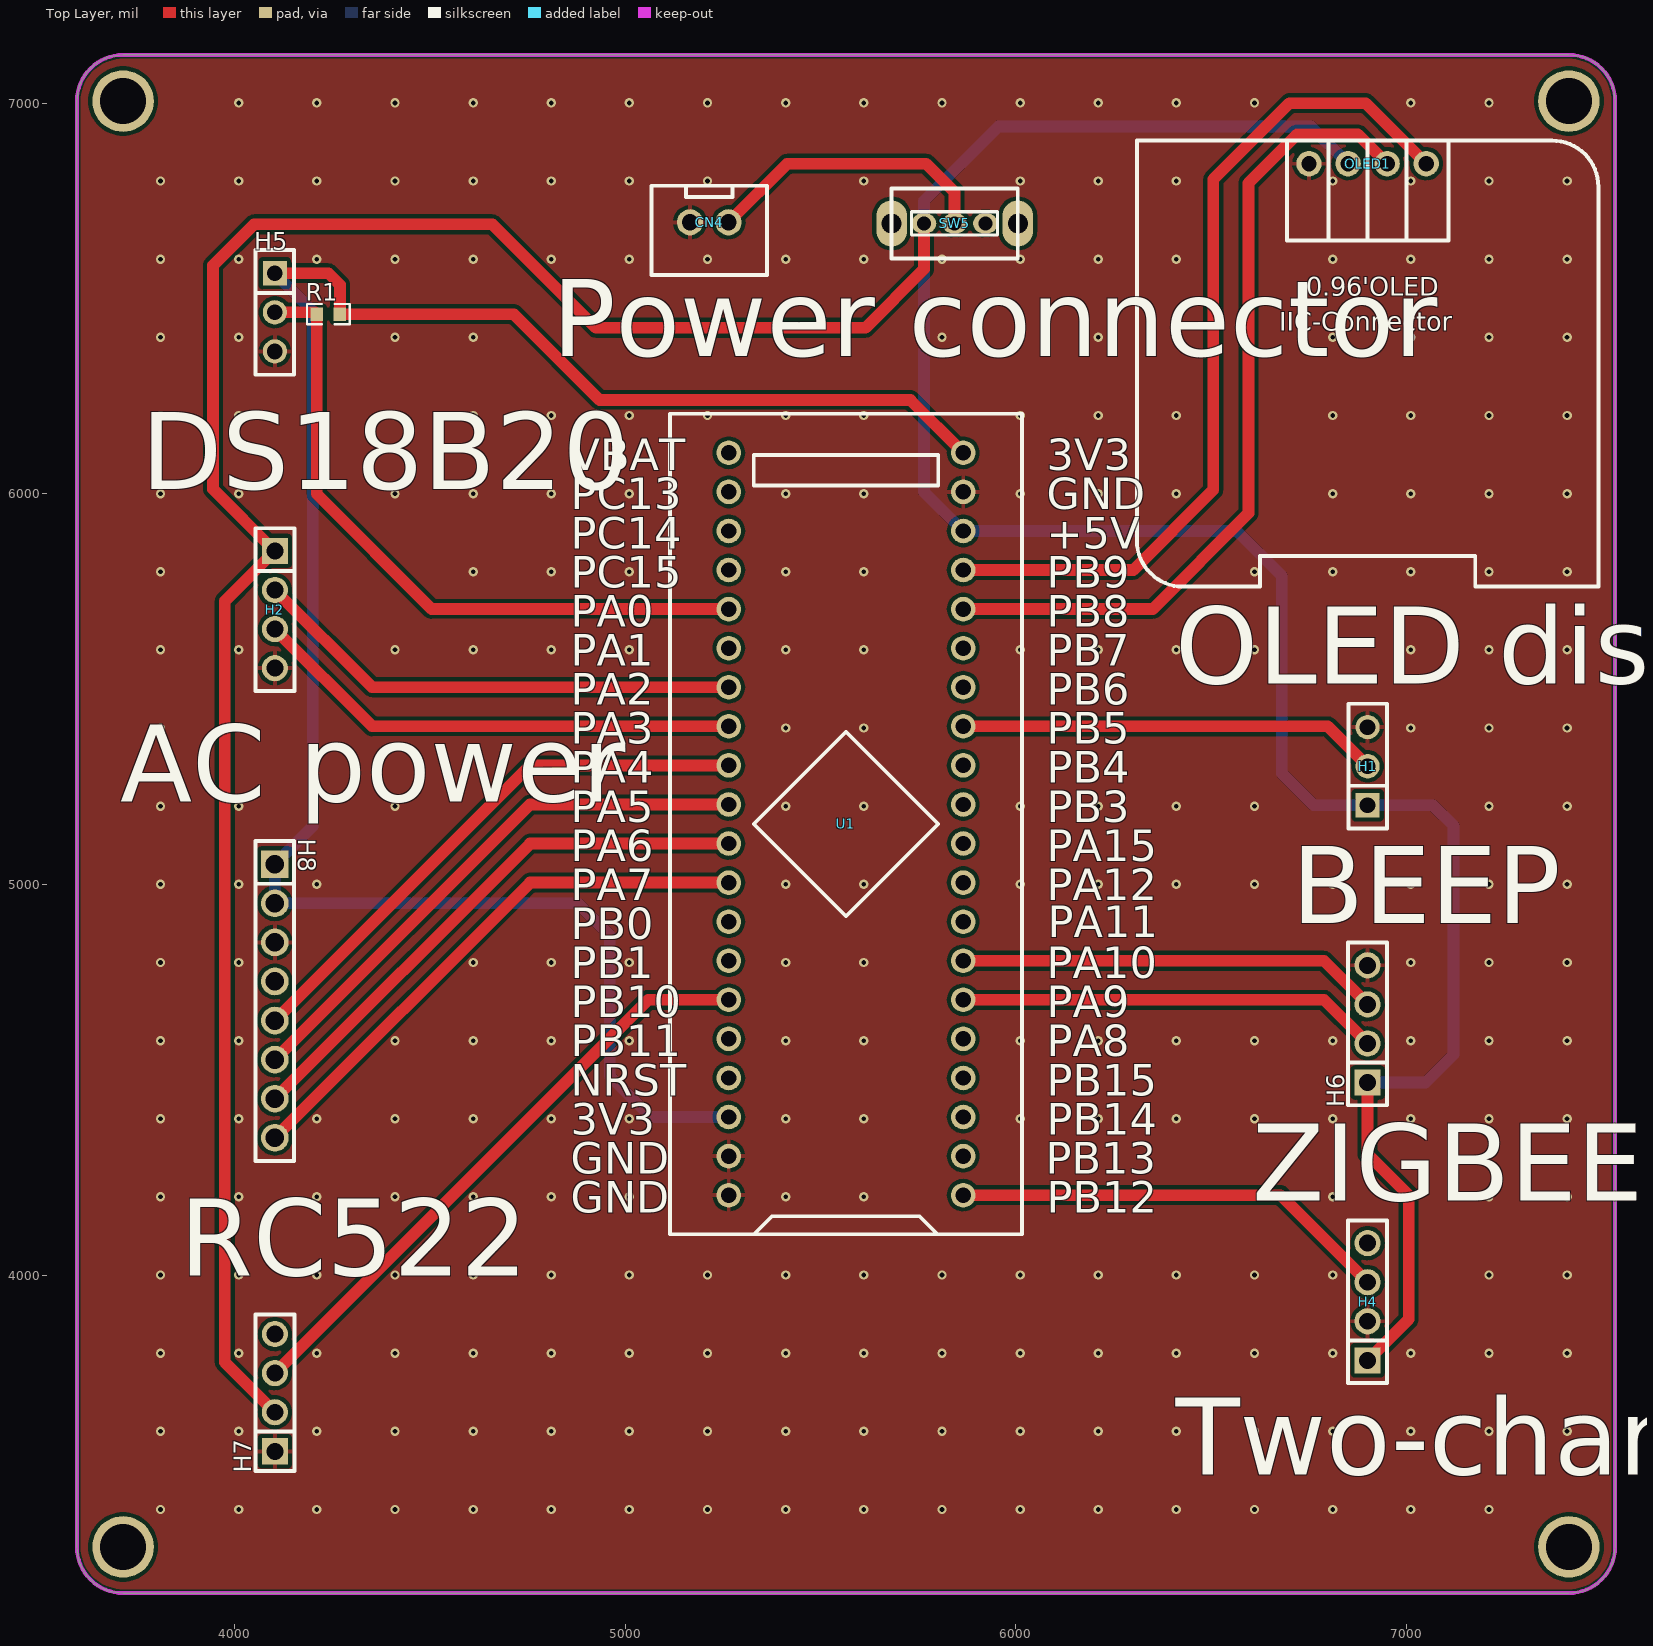
[diagram p0: Top Layer view]
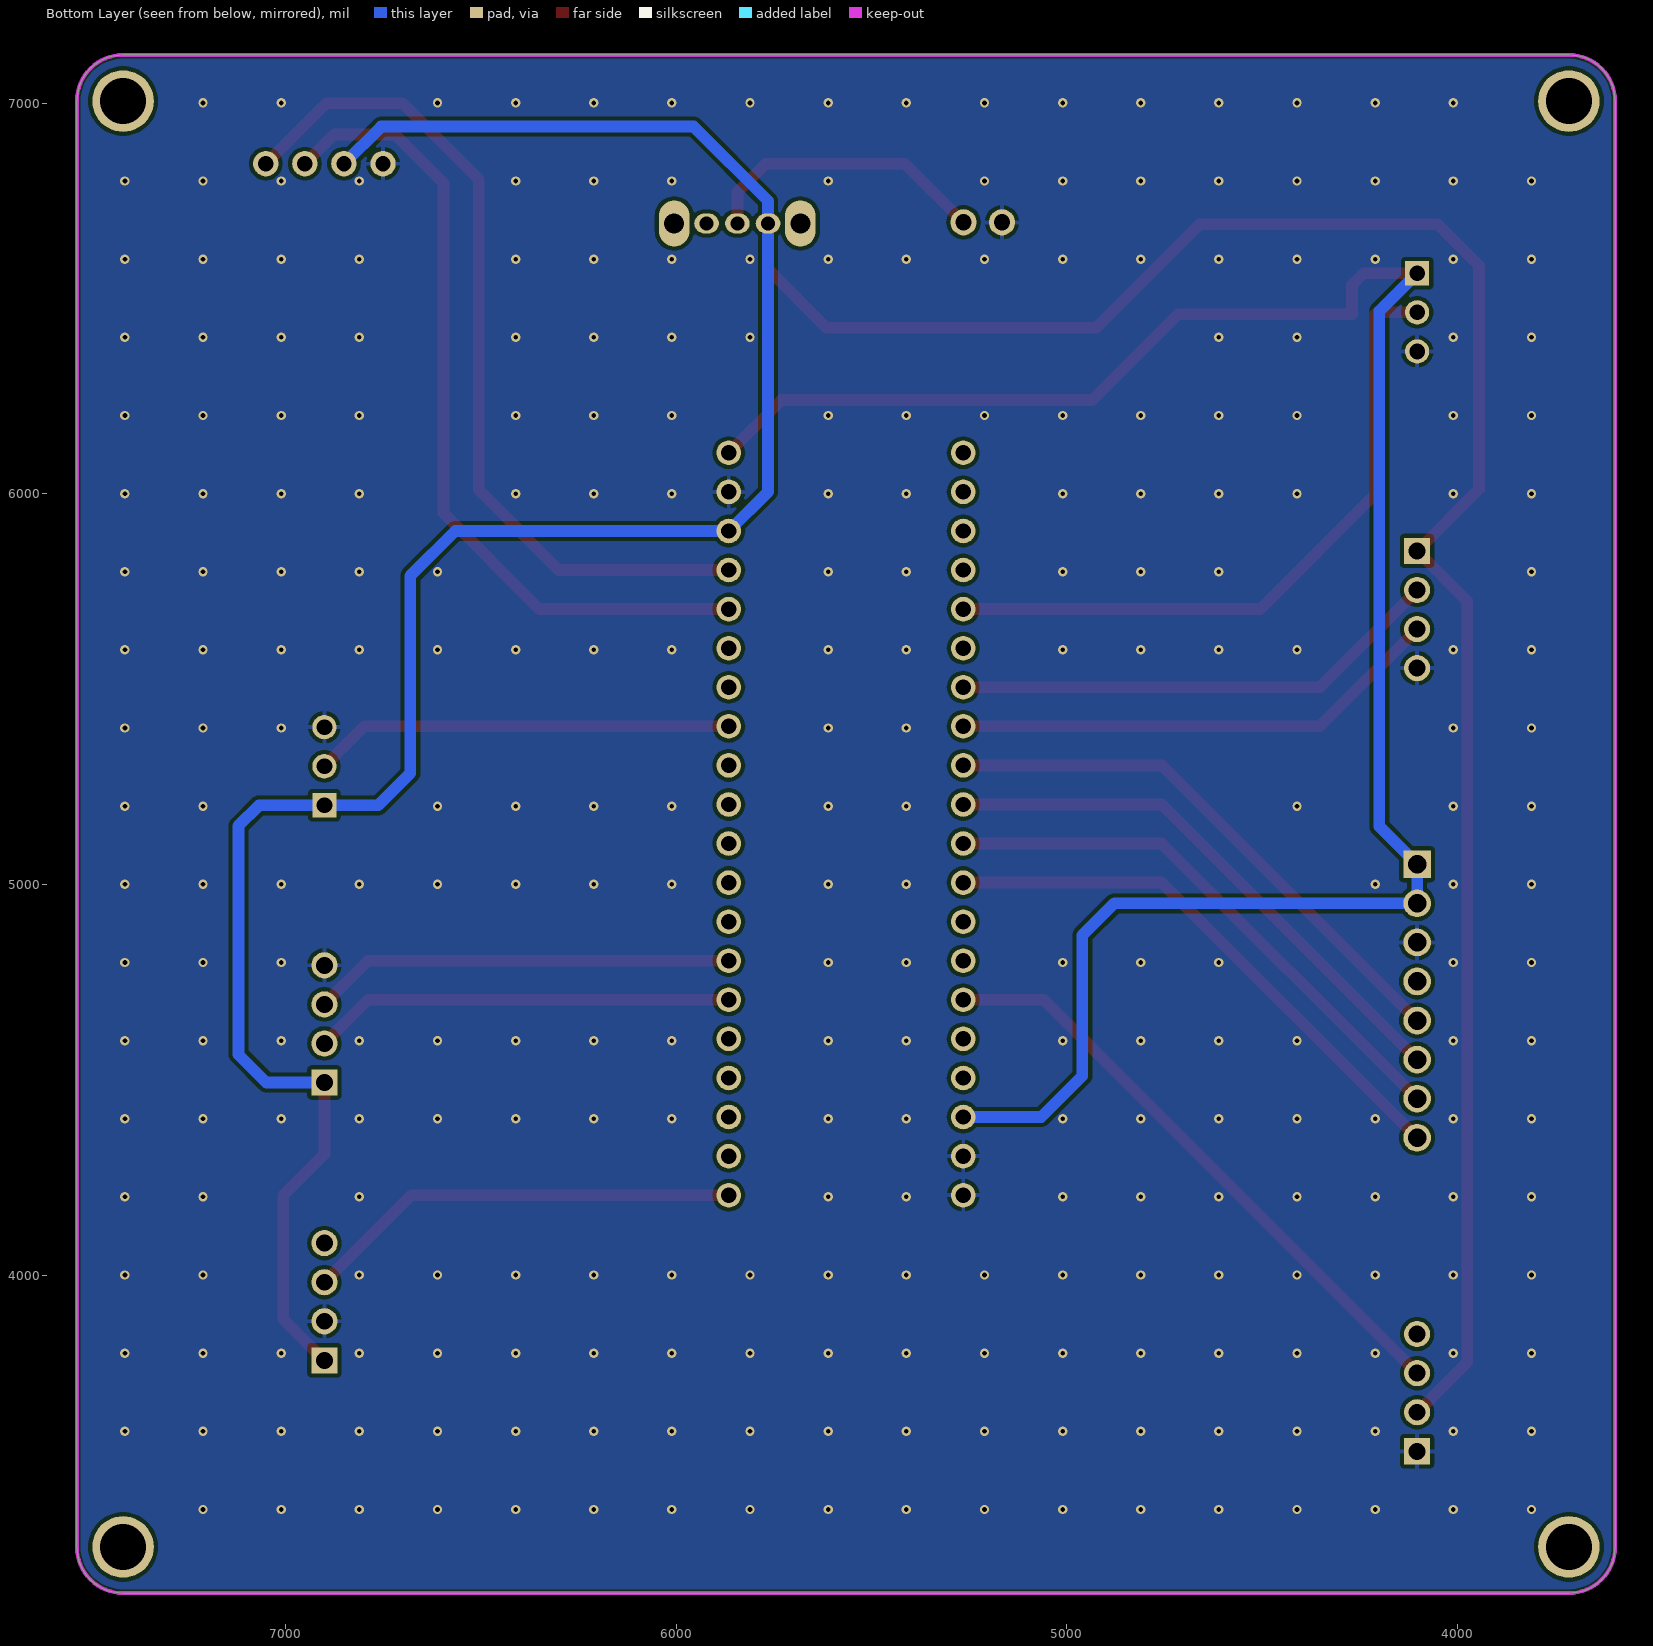
[diagram p1: Bottom Layer view, seen from below]
# Altium PCB MISC88997.pcbdoc
Units mil, origin at the board's own origin, x right, y up, seen from the top; angles counter-clockwise.
Board outline 3937.01 x 3937.01 mil, 2 copper layers (Top Layer, Bottom Layer), stack 62.206 mil thick; 12 components, 38 nets, 87 pads, 280 vias.

## Layer stack, top to bottom
Top Solder Mask Layer: solder mask 0.394, Dk 3.3
Top Layer: signal copper 1.379
Dielectric1: surface 59.449, FR4, Dk 4.5
Bottom Layer: signal copper 1.378
Bottom Solder Mask Layer: solder mask 0.394, Dk 3.3

## Board outline
3714.61,7123.5 ccw(c3714.61,7005.39) 3596.5,7005.39 3596.5,3304.61 ccw(c3714.61,3304.61) 3714.61,3186.5 7415.39,3186.5 ccw(c7415.39,3304.61) 7533.5,3304.61 7533.5,7005.39 ccw(c7415.39,7005.39) 7415.39,7123.5 3714.61,7123.5

## Design rules (kind name [scope] priority, off if disabled: settings)
BoardOutlineClearance copperThickness2oz_1 [All] p2 off: genericclearance=7.99 ignorepadtopadclearanceinfootprint=FALSE except(0: Arc-SplitContinuation Track-SplitContinuation SMDPad-SplitContinuation THPad-SplitContinuation Via-SplitContinuation Fill-SplitContinuation Region-SplitContinuation Poly-SplitContinuation Text-SplitContinuation Hole-SplitContinuation; 5.98: Arc-CutoutEdge Track-CutoutEdge SMDPad-CutoutEdge THPad-CutoutEdge Via-CutoutEdge Text-CutoutEdge; 6.9: Hole-OutlineEdge Hole-CutoutEdge; 10: Poly-OutlineEdge Poly-CutoutEdge; 11.81: Arc-OutlineEdge Track-OutlineEdge SMDPad-OutlineEdge THPad-OutlineEdge Via-OutlineEdge Fill-OutlineEdge Region-OutlineEdge Text-OutlineEdge Fill-CutoutEdge Region-CutoutEdge)
BoardOutlineClearance Plane_innerPlane_1 [All] p4 off: genericclearance=4.02 ignorepadtopadclearanceinfootprint=FALSE except(0: Arc-SplitContinuation Track-SplitContinuation SMDPad-SplitContinuation THPad-SplitContinuation Via-SplitContinuation Fill-SplitContinuation Region-SplitContinuation Poly-SplitContinuation Text-SplitContinuation Hole-SplitContinuation; 5.98: Arc-CutoutEdge Track-CutoutEdge SMDPad-CutoutEdge THPad-CutoutEdge Via-CutoutEdge Text-CutoutEdge; 6.9: Hole-OutlineEdge Hole-CutoutEdge; 10: Poly-OutlineEdge Poly-CutoutEdge; 11.81: Arc-OutlineEdge Track-OutlineEdge SMDPad-OutlineEdge THPad-OutlineEdge Via-OutlineEdge Fill-OutlineEdge Region-OutlineEdge Text-OutlineEdge Fill-CutoutEdge Region-CutoutEdge)
BoardOutlineClearance Copper_copperRegion_1 [All] p6 off: genericclearance=4.02 ignorepadtopadclearanceinfootprint=FALSE except(0: Arc-SplitContinuation Track-SplitContinuation SMDPad-SplitContinuation THPad-SplitContinuation Via-SplitContinuation Fill-SplitContinuation Region-SplitContinuation Poly-SplitContinuation Text-SplitContinuation Hole-SplitContinuation; 5.98: Arc-CutoutEdge Track-CutoutEdge SMDPad-CutoutEdge THPad-CutoutEdge Via-CutoutEdge Text-CutoutEdge; 6.9: Hole-OutlineEdge Hole-CutoutEdge; 10: Poly-OutlineEdge Poly-CutoutEdge; 11.81: Arc-OutlineEdge Track-OutlineEdge SMDPad-OutlineEdge THPad-OutlineEdge Via-OutlineEdge Fill-OutlineEdge Region-OutlineEdge Text-OutlineEdge Fill-CutoutEdge Region-CutoutEdge)
BoardOutlineClearance Copper_copperRegion_copperThickness1oz_1 [All] p8 off: genericclearance=4.02 ignorepadtopadclearanceinfootprint=FALSE except(0: Arc-SplitContinuation Track-SplitContinuation SMDPad-SplitContinuation THPad-SplitContinuation Via-SplitContinuation Fill-SplitContinuation Region-SplitContinuation Poly-SplitContinuation Text-SplitContinuation Hole-SplitContinuation; 5.98: Arc-CutoutEdge Track-CutoutEdge SMDPad-CutoutEdge THPad-CutoutEdge Via-CutoutEdge Text-CutoutEdge; 6.9: Hole-OutlineEdge Hole-CutoutEdge; 10: Poly-OutlineEdge Poly-CutoutEdge; 11.81: Arc-OutlineEdge Track-OutlineEdge SMDPad-OutlineEdge THPad-OutlineEdge Via-OutlineEdge Fill-OutlineEdge Region-OutlineEdge Text-OutlineEdge Fill-CutoutEdge Region-CutoutEdge)
BoardOutlineClearance Copper_copperRegion_Copper_copperRegion_1 [All] p10 off: genericclearance=4.02 ignorepadtopadclearanceinfootprint=FALSE except(0: Arc-SplitContinuation Track-SplitContinuation SMDPad-SplitContinuation THPad-SplitContinuation Via-SplitContinuation Fill-SplitContinuation Region-SplitContinuation Poly-SplitContinuation Text-SplitContinuation Hole-SplitContinuation; 5.98: Arc-CutoutEdge Track-CutoutEdge SMDPad-CutoutEdge THPad-CutoutEdge Via-CutoutEdge Text-CutoutEdge; 6.9: Hole-OutlineEdge Hole-CutoutEdge; 10: Poly-OutlineEdge Poly-CutoutEdge; 11.81: Arc-OutlineEdge Track-OutlineEdge SMDPad-OutlineEdge THPad-OutlineEdge Via-OutlineEdge Fill-OutlineEdge Region-OutlineEdge Text-OutlineEdge Fill-CutoutEdge Region-CutoutEdge)
BoardOutlineClearance copperThickness1oz_1 [All] p12: genericclearance=4.02 ignorepadtopadclearanceinfootprint=FALSE except(0: Arc-SplitContinuation Track-SplitContinuation SMDPad-SplitContinuation THPad-SplitContinuation Via-SplitContinuation Fill-SplitContinuation Region-SplitContinuation Poly-SplitContinuation Text-SplitContinuation Hole-SplitContinuation; 5.98: Arc-CutoutEdge Track-CutoutEdge SMDPad-CutoutEdge THPad-CutoutEdge Via-CutoutEdge Text-CutoutEdge; 6.9: Hole-OutlineEdge Hole-CutoutEdge; 10: Poly-OutlineEdge Poly-CutoutEdge; 11.81: Arc-OutlineEdge Track-OutlineEdge SMDPad-OutlineEdge THPad-OutlineEdge Via-OutlineEdge Fill-OutlineEdge Region-OutlineEdge Text-OutlineEdge Fill-CutoutEdge Region-CutoutEdge)
Clearance copperThickness2oz [All] p1 off: gap=7.99 ignorepadtopadclearanceinfootprint=FALSE except(5.98: SMDPad-Track SMDPad-SMDPad THPad-Track SMDPad-THPad THPad-THPad Track-Via SMDPad-Via THPad-Via Via-Via Fill-SMDPad Region-SMDPad Fill-THPad Region-THPad Fill-Via Region-Via Fill-Fill Fill-Region Region-Region Arc-Track Arc-SMDPad Arc-THPad Arc-Via Fill-Arc Region-Arc Arc-Arc Text-Track SMDPad-Text Text-THPad Text-Via Fill-Text Region-Text Arc-Text Text-Text; 6.9: Hole-Track Hole-SMDPad Hole-THPad Hole-Via Fill-Hole Region-Hole Hole-Arc Hole-Text; 10: Poly-Track Poly-SMDPad Poly-THPad Poly-Via Poly-Fill Poly-Region Poly-Poly Poly-Arc Poly-Text Poly-Hole; 11.81: Fill-Track Region-Track)
Clearance Plane_innerPlane [All] p3 off: gap=4.02 ignorepadtopadclearanceinfootprint=FALSE except(5.98: SMDPad-Track SMDPad-SMDPad THPad-Track SMDPad-THPad THPad-THPad Track-Via SMDPad-Via THPad-Via Via-Via Fill-SMDPad Region-SMDPad Fill-THPad Region-THPad Fill-Via Region-Via Fill-Fill Fill-Region Region-Region Arc-Track Arc-SMDPad Arc-THPad Arc-Via Fill-Arc Region-Arc Arc-Arc Text-Track SMDPad-Text Text-THPad Text-Via Fill-Text Region-Text Arc-Text Text-Text; 6.9: Hole-Track Hole-SMDPad Hole-THPad Hole-Via Fill-Hole Region-Hole Hole-Arc Hole-Text; 10: Poly-Track Poly-SMDPad Poly-THPad Poly-Via Poly-Fill Poly-Region Poly-Poly Poly-Arc Poly-Text Poly-Hole; 11.81: Fill-Track Region-Track)
Clearance Copper_copperRegion [All] p5 off: gap=4.02 ignorepadtopadclearanceinfootprint=FALSE except(5.98: SMDPad-Track SMDPad-SMDPad THPad-Track SMDPad-THPad THPad-THPad Track-Via SMDPad-Via THPad-Via Via-Via Fill-SMDPad Region-SMDPad Fill-THPad Region-THPad Fill-Via Region-Via Fill-Fill Fill-Region Region-Region Arc-Track Arc-SMDPad Arc-THPad Arc-Via Fill-Arc Region-Arc Arc-Arc Text-Track SMDPad-Text Text-THPad Text-Via Fill-Text Region-Text Arc-Text Text-Text; 6.9: Hole-Track Hole-SMDPad Hole-THPad Hole-Via Fill-Hole Region-Hole Hole-Arc Hole-Text; 10: Poly-Track Poly-SMDPad Poly-THPad Poly-Via Poly-Fill Poly-Region Poly-Poly Poly-Arc Poly-Text Poly-Hole; 11.81: Fill-Track Region-Track)
Clearance Copper_copperRegion_copperThickness1oz [All] p7 off: gap=4.02 ignorepadtopadclearanceinfootprint=FALSE except(5.98: SMDPad-Track SMDPad-SMDPad THPad-Track SMDPad-THPad THPad-THPad Track-Via SMDPad-Via THPad-Via Via-Via Fill-SMDPad Region-SMDPad Fill-THPad Region-THPad Fill-Via Region-Via Fill-Fill Fill-Region Region-Region Arc-Track Arc-SMDPad Arc-THPad Arc-Via Fill-Arc Region-Arc Arc-Arc Text-Track SMDPad-Text Text-THPad Text-Via Fill-Text Region-Text Arc-Text Text-Text; 6.9: Hole-Track Hole-SMDPad Hole-THPad Hole-Via Fill-Hole Region-Hole Hole-Arc Hole-Text; 10: Poly-Track Poly-SMDPad Poly-THPad Poly-Via Poly-Fill Poly-Region Poly-Poly Poly-Arc Poly-Text Poly-Hole; 11.81: Fill-Track Region-Track)
Clearance Copper_copperRegion_Copper_copperRegion [All] p9 off: gap=4.02 ignorepadtopadclearanceinfootprint=FALSE except(5.98: SMDPad-Track SMDPad-SMDPad THPad-Track SMDPad-THPad THPad-THPad Track-Via SMDPad-Via THPad-Via Via-Via Fill-SMDPad Region-SMDPad Fill-THPad Region-THPad Fill-Via Region-Via Fill-Fill Fill-Region Region-Region Arc-Track Arc-SMDPad Arc-THPad Arc-Via Fill-Arc Region-Arc Arc-Arc Text-Track SMDPad-Text Text-THPad Text-Via Fill-Text Region-Text Arc-Text Text-Text; 6.9: Hole-Track Hole-SMDPad Hole-THPad Hole-Via Fill-Hole Region-Hole Hole-Arc Hole-Text; 10: Poly-Track Poly-SMDPad Poly-THPad Poly-Via Poly-Fill Poly-Region Poly-Poly Poly-Arc Poly-Text Poly-Hole; 11.81: Fill-Track Region-Track)
Clearance copperThickness1oz [All] p11: gap=4.02 ignorepadtopadclearanceinfootprint=FALSE except(5.98: SMDPad-Track SMDPad-SMDPad THPad-Track SMDPad-THPad THPad-THPad Track-Via SMDPad-Via THPad-Via Via-Via Fill-SMDPad Region-SMDPad Fill-THPad Region-THPad Fill-Via Region-Via Fill-Fill Fill-Region Region-Region Arc-Track Arc-SMDPad Arc-THPad Arc-Via Fill-Arc Region-Arc Arc-Arc Text-Track SMDPad-Text Text-THPad Text-Via Fill-Text Region-Text Arc-Text Text-Text; 6.9: Hole-Track Hole-SMDPad Hole-THPad Hole-Via Fill-Hole Region-Hole Hole-Arc Hole-Text; 10: Poly-Track Poly-SMDPad Poly-THPad Poly-Via Poly-Fill Poly-Region Poly-Poly Poly-Arc Poly-Text Poly-Hole; 11.81: Fill-Track Region-Track)
DiffPairsRouting differentialPair [All] p1: maxlimit=6 minlimit=6 mostfreqgap=6 toplayer_minwidth=5 toplayer_prefwidth=10 toplayer_maxwidth=100 toplayer_mingap=6 toplayer_prefgap=6 toplayer_maxgap=6 bottomlayer_minwidth=5 bottomlayer_prefwidth=10 bottomlayer_maxwidth=100 bottomlayer_mingap=6 bottomlayer_prefgap=6 bottomlayer_maxgap=6 maxuncoupledlength=10
HoleToHoleClearance otherClearance [All] p1: gap=11.81 allowstackedmicrovias=TRUE
Length netLength [All] p1: minlimit=0 maxlimit=0
PasteMaskExpansion pasteMaskExpansion [All] p1: expansion=0
PlaneConnect innerPlane [All] p1: planeconnectstyle=Relief reliefexpansion=20 reliefentries=4 reliefconductorwidth=10 reliefairgap=10
PolygonConnect copperRegion_copperThickness1oz [All] p1 off: connectstyle=Relief reliefconductorwidth=10 reliefentries=4 polygonreliefangle="90 Angle" airgapwidth=10 via.connectstyle=Relief via.reliefconductorwidth=10 via.reliefentries=4 via.polygonreliefangle="90 Angle" via.airgapwidth=10
PolygonConnect copperRegion_Copper_copperRegion [All] p2 off: connectstyle=Relief reliefconductorwidth=10 reliefentries=4 polygonreliefangle="90 Angle" airgapwidth=10 via.connectstyle=Relief via.reliefconductorwidth=10 via.reliefentries=4 via.polygonreliefangle="90 Angle" via.airgapwidth=10
PolygonConnect copperRegion [All] p3: connectstyle=Relief reliefconductorwidth=10 reliefentries=4 polygonreliefangle="90 Angle" airgapwidth=10 via.connectstyle=Relief via.reliefconductorwidth=10 via.reliefentries=4 via.polygonreliefangle="90 Angle" via.airgapwidth=10
RoutingVias viaSize [All] p1: holewidth=12.01 width=24.02 viastyle="Through Hole" minholewidth=11.81 minwidth=19.68 maxholewidth=248.03 maxwidth=393.7
SolderMaskExpansion solderMaskExpansion [IsVia] p1: expansion=-1000 istentingtop=TRUE
SolderMaskExpansion solderMaskExpansion [All] p2: expansion=2 istentingtop=FALSE
Width copperThickness2oz_2 [All] p1 off: maxlimit=100 minlimit=8 preferedwidth=10
Width copperThickness1oz_2 [All] p2: maxlimit=100 minlimit=5 preferedwidth=10

## Components (designator, comment, footprint, x,y, rotation, side; value= is the part's Value field where it differs from the comment)
CN4 "XH2.54*2P_through-hole" CONN-TH_2P-P2.50-XH2.54-2P 5215,6695 r0 top
H1 "" HDR-TH_3P-P2.54-V-F 6900,5302.82 r90 top
H2 "" HDR-TH_4P-P2.54-V-F 4103.27,5703.79 r270 top
H4 "" HDR-TH_4P-P2.54-V-F 6900,3932.22 r90 top
H5 "" HDR-TH_3P-P2.54-V-F 4103.27,6464.57 r270 top
H6 "" HDR-TH_4P-P2.54-V-F 6900,4643.38 r90 top
H7 "" HDR-TH_4P-P2.54-V-M 4103.27,3699.44 r90 top
H8 "" HDR-TH_8P-P2.54-V-F-1 4103.27,4701.96 r270 top
OLED1 "" 0.96OLED_4P 6900,6845 r0 top
R1 "4.7K" R0603 4240,6460 r0 top
SW5 "" 拨动开关 5837.9,6692.05 r0 top
U1 "STM32F103C8T6-Card" CONN-TH_L53.3-W22.9_STM32F103C8T6-CARD 5565,5155 r90 top

## Footprints (in the part's own frame and the unit in brackets; to place one, negate y for a bottom-side part, rotate by r counter-clockwise, add the part's x,y. Pads: shape width x height; smd on the part's side, far side on the other; paste and mask are expansions set on the pad)
0.96OLED_4P [mm]
  round 1.65 hole 1 copper offset 0,0: 1(-3.81,-0.001) 2(-1.27,0.002) 3(1.27,0.002) 4(3.81,0.002)
  silkscreen extent -15,-27.5 15,1.5
CONN-TH_2P-P2.50-XH2.54-2P [mm]
  round 1.7 hole 1.05 paste+0 mask+0.05: 1(1.25,0) 2(-1.25,0)
  silkscreen extent -3.75,-3.42 3.75,2.37
CONN-TH_L53.3-W22.9_STM32F103C8T6-CARD [mm]
  round 1.6 hole 1: 1(-24.13,-7.62) 2(-21.59,-7.62) 3(-19.05,-7.62) 4(-16.51,-7.62) 5(-13.97,-7.62) 6(-11.43,-7.62) 7(-8.89,-7.62) 8(-6.35,-7.62) 9(-3.81,-7.62) 10(-1.27,-7.62) 11(1.27,-7.62) 12(3.81,-7.62) 13(6.35,-7.62) 14(8.89,-7.62) 15(11.43,-7.62) 16(13.97,-7.62) 17(16.51,-7.62) 18(19.05,-7.62) 19(21.59,-7.62) 20(24.13,-7.62) 21(24.13,7.62) 22(21.59,7.62) 23(19.05,7.62) 24(16.51,7.62) 25(13.97,7.62) 26(11.43,7.62) 27(8.89,7.62) 28(6.35,7.62) 29(3.81,7.62) 30(1.27,7.62) 31(-1.27,7.62) 32(-3.81,7.62) 33(-6.35,7.62) 34(-8.89,7.62) 35(-11.43,7.62) 36(-13.97,7.62) 37(-16.51,7.62) 38(-19.05,7.62) 39(-21.59,7.62) 40(-24.13,7.62)
  silkscreen extent -26.67,-11.43 26.67,11.43
HDR-TH_3P-P2.54-V-F [mil]
  rect 62x62 hole 40.16: 1(-100,0)
  round 62 hole 40.16: 2(0,0) 3(100,0)
  silkscreen extent -160,-49 160,49
HDR-TH_4P-P2.54-V-F [mm]
  rect 1.7x1.7 hole 1.1: 1(-3.81,0)
  round 1.7 hole 1.1: 2(-1.27,0) 3(1.27,0) 4(3.81,0)
  silkscreen extent -5.29,-1.27 5.29,1.27
HDR-TH_4P-P2.54-V-M [mm]
  rect 1.7x1.7 hole 1.1: 1(-3.81,0)
  round 1.7 hole 1.1: 2(-1.27,0) 3(1.27,0) 4(3.81,0)
  silkscreen extent -5.08,-1.27 5.08,1.27
HDR-TH_8P-P2.54-V-F-1 [mm]
  rect 1.8x1.8 hole 1.2: 1(-8.89,0)
  round 1.8 hole 1.2: 2(-6.35,0) 3(-3.81,0) 4(-1.27,0) 5(1.27,0) 6(3.81,0) 7(6.35,0) 8(8.89,0)
  silkscreen extent -10.41,-1.25 10.41,1.25
R0603 [mil]
  rect 31.75x34.02 smd paste-3937.01 mask+2: 1(-29.66,0) 2(29.66,0)
  silkscreen extent -55,-26 55,26
拨动开关 [mil]
  oval 63x51.2 hole 35.4 paste+0 mask+2: 1(-73.4,0) 2(5,0) 3(84,0)
  oval 78.7x118.1 hole 51.2 paste+0 mask+2: 4(166.7,0) 5(-156.1,0)
  silkscreen extent -156,-90 167,90

## Free pads (board coordinates)
  round 157.48 hole 118.11: 1(3714.61,7005.39) 1(3714.61,3304.61) 1(7415.39,7005.39) 1(7415.39,3304.61)

## Via types
v1: diameter 24.02, hole 12, Top Layer to Bottom Layer, 280 vias

## Nets (pads, with @x,y where several pads share a name; then routed paths per layer and width w, separated by ;. In a path a pad name is that pad's centre, name@x,y a point inside that pad or via, vN(x,y) a via of type N, cw(c..) or ccw(c..) an arc to the next point about the centre after c; other vN are vias at no path point)
$1N17118: CN4.1 SW5.2 | length 751.1
  Top Layer w30: CN4.1 5414.22,6845 5770,6845 5842.9,6772.1 SW5.2
+5V: H1.1 H2.1 H4.1 H6.1 H7.2 OLED1.2 SW5.1 U1.18 | length 10845.8
  Top Layer w30: H7.2 3975,3777.71 3975,5725.52 H2.1 3945,6012.05 3945,6585 4050,6690 4660,6690 4925,6425 5615,6425 5764.5,6574.5 SW5.1 ; H4.1 7005,3887.23 7005,4205 6900,4310 H6.1
  Bottom Layer w30: OLED1.2@6850,6845.05 6755.05,6940 5955,6940 5764.5,6749.5 SW5.1 5764.5,6005.5 U1.18 6565,5905 6680,5790 6680,5285 6762.18,5202.82 H1.1 7067.18,5202.82 7120,5150 7120,4565 7048.38,4493.38 H6.1
GND: CN4.2 H1.3 H2.4 H4.2 H5.3 H6.4 H7.1 H8.3 OLED1.1 U1.19 U1.39 U1.40
  other v1: 3810.6,3400.6 4010.6,3400.6 4210.6,3400.6 4410.6,3400.6 4610.6,3400.6 4810.6,3400.6 5010.6,3400.6 5210.6,3400.6 5410.6,3400.6 5610.6,3400.6 5810.6,3400.6 6010.6,3400.6 6210.6,3400.6 6410.6,3400.6 6610.6,3400.6 6810.6,3400.6 7010.6,3400.6 7210.6,3400.6 3810.6,3600.6 4010.6,3600.6 4210.6,3600.6 4410.6,3600.6 4610.6,3600.6 4810.6,3600.6 5010.6,3600.6 5210.6,3600.6 5410.6,3600.6 5610.6,3600.6 5810.6,3600.6 6010.6,3600.6 6210.6,3600.6 6410.6,3600.6 6610.6,3600.6 6810.6,3600.6 7010.6,3600.6 7210.6,3600.6 7410.6,3600.6 3810.6,3800.6 4010.6,3800.6 4210.6,3800.6 4410.6,3800.6 4610.6,3800.6 4810.6,3800.6 5010.6,3800.6 5210.6,3800.6 5410.6,3800.6 5610.6,3800.6 5810.6,3800.6 6010.6,3800.6 6210.6,3800.6 6410.6,3800.6 6610.6,3800.6 6810.6,3800.6 7010.6,3800.6 7210.6,3800.6 7410.6,3800.6 3810.6,4000.6 4010.6,4000.6 4210.6,4000.6 4410.6,4000.6 4610.6,4000.6 4810.6,4000.6 5010.6,4000.6 5210.6,4000.6 5410.6,4000.6 5610.6,4000.6 5810.6,4000.6 6010.6,4000.6 6210.6,4000.6 6410.6,4000.6 6610.6,4000.6 6810.6,4000.6 7210.6,4000.6 7410.6,4000.6 3810.6,4200.6 4010.6,4200.6 4210.6,4200.6 4410.6,4200.6 4610.6,4200.6 4810.6,4200.6 5010.6,4200.6 5410.6,4200.6 5610.6,4200.6 6810.6,4200.6 7210.6,4200.6 7410.6,4200.6 3810.6,4400.6 4010.6,4400.6 4210.6,4400.6 4410.6,4400.6 4610.6,4400.6 4810.6,4400.6 5010.6,4400.6 5410.6,4400.6 5610.6,4400.6 6010.6,4400.6 6210.6,4400.6 6410.6,4400.6 6610.6,4400.6 6810.6,4400.6 7010.6,4400.6 7210.6,4400.6 7410.6,4400.6 3810.6,4600.6 4010.6,4600.6 4410.6,4600.6 4610.6,4600.6 4810.6,4600.6 5010.6,4600.6 5410.6,4600.6 5610.6,4600.6 6010.6,4600.6 6210.6,4600.6 6410.6,4600.6 6610.6,4600.6 6810.6,4600.6 7010.6,4600.6 7210.6,4600.6 7410.6,4600.6 3810.6,4800.6 4010.6,4800.6 4610.6,4800.6 4810.6,4800.6 5010.6,4800.6 5410.6,4800.6 5610.6,4800.6 7010.6,4800.6 7210.6,4800.6 7410.6,4800.6 3810.6,5000.6 4010.6,5000.6 4210.6,5000.6 5410.6,5000.6 5610.6,5000.6 6010.6,5000.6 6210.6,5000.6 6410.6,5000.6 6610.6,5000.6 6810.6,5000.6 7010.6,5000.6 7210.6,5000.6 7410.6,5000.6 3810.6,5200.6 4010.6,5200.6 4410.6,5200.6 5410.6,5200.6 5610.6,5200.6 6010.6,5200.6 6210.6,5200.6 6410.6,5200.6 6610.6,5200.6 7210.6,5200.6 7410.6,5200.6 3810.6,5400.6 4010.6,5400.6 5410.6,5400.6 5610.6,5400.6 7010.6,5400.6 7210.6,5400.6 7410.6,5400.6 3810.6,5600.6 4010.6,5600.6 4410.6,5600.6 4610.6,5600.6 4810.6,5600.6 5010.6,5600.6 5410.6,5600.6 5610.6,5600.6 6010.6,5600.6 6210.6,5600.6 6410.6,5600.6 6610.6,5600.6 6810.6,5600.6 7010.6,5600.6 7210.6,5600.6 7410.6,5600.6 3810.6,5800.6 4610.6,5800.6 4810.6,5800.6 5010.6,5800.6 5410.6,5800.6 5610.6,5800.6 6610.6,5800.6 6810.6,5800.6 7010.6,5800.6 7210.6,5800.6 7410.6,5800.6 3810.6,6000.6 4010.6,6000.6 4410.6,6000.6 4610.6,6000.6 4810.6,6000.6 5010.6,6000.6 5410.6,6000.6 5610.6,6000.6 6010.6,6000.6 6210.6,6000.6 6410.6,6000.6 6810.6,6000.6 7010.6,6000.6 7210.6,6000.6 7410.6,6000.6 3810.6,6200.6 4010.6,6200.6 4410.6,6200.6 4610.6,6200.6 4810.6,6200.6 5010.6,6200.6 5210.6,6200.6 5410.6,6200.6 5610.6,6200.6 6010.6,6200.6 6210.6,6200.6 6410.6,6200.6 6810.6,6200.6 7010.6,6200.6 7210.6,6200.6 7410.6,6200.6 3810.6,6400.6 4010.6,6400.6 4410.6,6400.6 4610.6,6400.6 5810.6,6400.6 6010.6,6400.6 6210.6,6400.6 6410.6,6400.6 6810.6,6400.6 7010.6,6400.6 7210.6,6400.6 7410.6,6400.6 3810.6,6600.6 4010.6,6600.6 4210.6,6600.6 4410.6,6600.6 4610.6,6600.6 4810.6,6600.6 5010.6,6600.6 5210.6,6600.6 5410.6,6600.6 5610.6,6600.6 5810.6,6600.6 6010.6,6600.6 6210.6,6600.6 6410.6,6600.6 6810.6,6600.6 7010.6,6600.6 7210.6,6600.6 7410.6,6600.6 3810.6,6800.6 4010.6,6800.6 4210.6,6800.6 4410.6,6800.6 4610.6,6800.6 4810.6,6800.6 5010.6,6800.6 5210.6,6800.6 5610.6,6800.6 6010.6,6800.6 6210.6,6800.6 6410.6,6800.6 6810.6,6800.6 7010.6,6800.6 7210.6,6800.6 7410.6,6800.6 4010.6,7000.6 4210.6,7000.6 4410.6,7000.6 4610.6,7000.6 4810.6,7000.6 5010.6,7000.6 5210.6,7000.6 5410.6,7000.6 5610.6,7000.6 5810.6,7000.6 6010.6,7000.6 6210.6,7000.6 6410.6,7000.6 6610.6,7000.6 7010.6,7000.6 7210.6,7000.6
MOSI: H8.6 U1.30 | length 1432.2
  Top Layer w30: H8.6 4756.31,5205 U1.30
MSO: H8.5 U1.29 | length 1432.2
  Top Layer w30: H8.5 4756.31,5305 U1.29
NRST: U1.37
PA0: H5.2 R1.1 U1.25 | length 1746
  Top Layer w30: H5.2 4205.77,6464.57 R1.1 4210.34,5999.66 4505,5705 U1.25
PA1: U1.26
PA2: H2.2 U1.27 | length 1264.8
  Top Layer w30: H2.2 4352.05,5505 U1.27
PA3: H2.3 U1.28 | length 1264.8
  Top Layer w30: H2.3 4352.05,5405 U1.28
PA8: U1.5
PA9: H6.2 U1.6 | length 1081.2
  Top Layer w30: U1.6 6788.37,4705 H6.2
PA10: H6.3 U1.7 | length 1081.2
  Top Layer w30: U1.7 6788.37,4805 H6.3
PA11: U1.8
PA12: U1.9
PA15: U1.10
PB0: U1.33
PB1: U1.34
PB3: U1.11
PB4: U1.12
PB5: H1.2 U1.13 | length 1077.3
  Top Layer w30: U1.13 6797.82,5405 H1.2
PB6: U1.14
PB7: U1.15
PB8: OLED1.3 U1.16 | length 2114.3
  Top Layer w30: U1.16 6350,5705 6595,5950 6595,6795 6720,6920 6875.05,6920 OLED1.3@6950,6845.05
PB9: OLED1.4 U1.17 | length 2209.9
  Top Layer w30: U1.17 6300,5805 6505,6010 6505,6805 6700,7000 6895.05,7000 OLED1.4@7050,6845.05
PB10: H7.3 U1.35 | length 1557.5
  Top Layer w30: H7.3 5058.82,4705 U1.35
PB11: U1.36
PB12: H4.3 U1.1 | length 1127.3
  Top Layer w30: U1.1 6677.21,4205 H4.3
PB13: U1.2
PB14: U1.3
PB15: U1.4
PC13: U1.22
PC14: U1.23
PC15: U1.24
SCK: H8.7 U1.31 | length 1432.2
  Top Layer w30: H8.7 4756.31,5105 U1.31
SDA: H8.8 U1.32 | length 1432.2
  Top Layer w30: H8.8 4756.31,5005 U1.32
VBAT: U1.21
VCC: H5.1 H8.1 H8.2 R1.2 U1.20 U1.38 | length 5288.1
  Top Layer w30: H5.1 4240.43,6564.57 4269.66,6535.34 R1.2 4715,6460 4935,6240 5730,6240 U1.20
  Bottom Layer w30: H5.1 4200,6467.83 4200,5148.69 H8.1 H8.2 4878.04,4951.96 4960,4870 4960,4510 5065,4405 U1.38
pads on no net: H4.4 H7.4 H8.4 SW5.3 SW5.4 SW5.5

## Polygon pours and split planes (outlines as drawn)
GND on Bottom Layer (solid, remove dead copper, pour order 2): 3525,7245 3525,3080 7700,3080 7700,7245
GND on Top Layer (solid, remove dead copper, pour order 2): 3000,7415 3000,3000 7930,3000 7930,7415

## Keep-outs
Board Outline Layer:
  the board outline again, w10

## Silkscreen, mask and mechanical layers (free items; w line width, h text height)
Top Silkscreen Layer:
  text "Power connector" at 4812.87,6351.57 h196.85
  text "VBAT" at 4860.95,6060 h80
  text "3V3" at 6079.16,6060 h80
  text "DS18B20" at 3761.16,6011.75 h196.85
  text "PC13" at 4860.95,5960 h80
  text "GND" at 6079.16,5960 h80
  text "PC14" at 4860.95,5860 h80
  text "+5V" at 6079.16,5860 h80
  text "PC15" at 4860.95,5760 h80
  text "PB9" at 6079.16,5760 h80
  text "PA0" at 4860.95,5660 h80
  text "PB8" at 6079.16,5660 h80
  text "PA1" at 4860.95,5560 h80
  text "PB7" at 6079.16,5560 h80
  text "OLED display" at 6408.02,5514.09 h196.85
  text "PA2" at 4860.95,5460 h80
  text "PB6" at 6079.16,5460 h80
  text "PA3" at 4860.95,5360 h80
  text "PB5" at 6079.16,5360 h80
  text "PA4" at 4860.95,5260 h80
  text "PB4" at 6079.16,5260 h80
  text "AC power" at 3708.07,5211.5 h196.85
  text "PA5" at 4860.95,5160 h80
  text "PB3" at 6079.16,5160 h80
  text "PA6" at 4860.95,5060 h80
  text "PA15" at 6079.16,5060 h80
  text "PA7" at 4860.95,4960 h80
  text "PA12" at 6079.16,4960 h80
  text "BEEP" at 6705.68,4900.68 h196.85
  text "PA11" at 6080.95,4865 h80
  text "PB0" at 4860.95,4860 h80
  text "PB1" at 4860.95,4760 h80
  text "PA10" at 6079.16,4760 h80
  text "PB10" at 4860.95,4660 h80
  text "PA9" at 6079.16,4660 h80
  text "PB11" at 4860.95,4560 h80
  text "PA8" at 6079.16,4560 h80
  text "NRST" at 4860.95,4460 h80
  text "PB15" at 6079.16,4460 h80
  text "3V3" at 4860.95,4360 h80
  text "PB14" at 6079.16,4360 h80
  text "GND" at 4860.95,4260 h80
  text "PB13" at 6075.95,4260 h80
  text "ZIGBEE" at 6604.57,4191.31 h196.85
  text "GND" at 4860.95,4160 h80
  text "PB12" at 6079.16,4160 h80
  text "RC522" at 3860.33,3999.14 h196.85
  text "Two-channel relay" at 6408.39,3490 h196.85